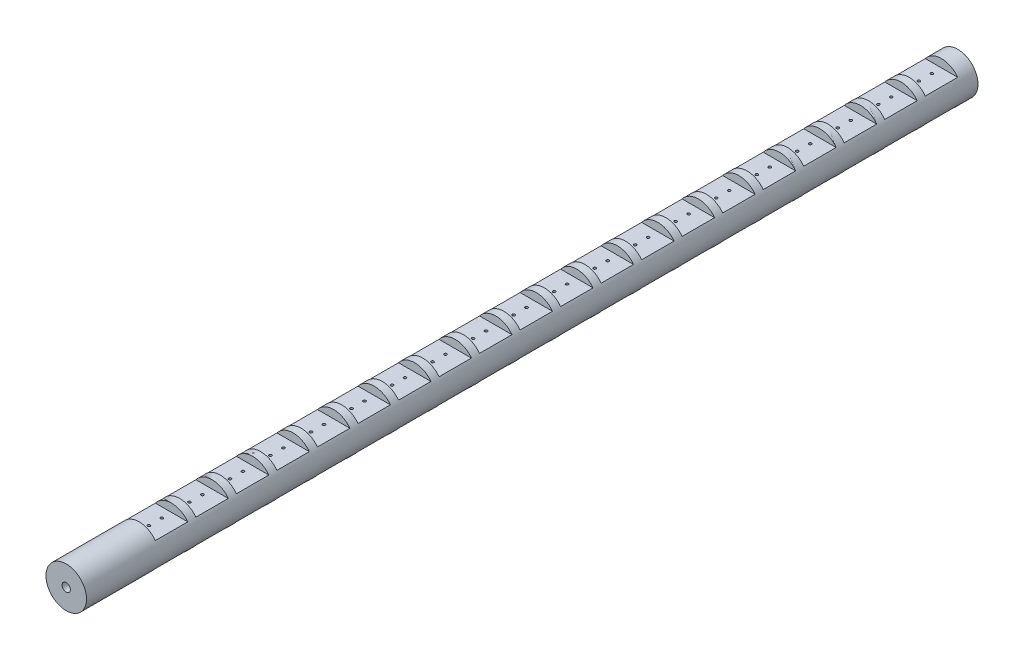
from build123d import *

# Parameters (mm, degrees)
SKETCH1_R                  = 25
BOSS_EXTRUDE1_DEPTH        = 1100
M12_TAPPED_HOLE1_D         = 10.2
M12_TAPPED_HOLE1_DEPTH     = 29.25
M12_TAPPED_HOLE1_TIP       = 3.064389157
SKETCH3_R                  = 10
CUT_EXTRUDE1_DEPTH         = 484
CUT_EXTRUDE2_START         = -15
SKETCH4_W                  = 50
SKETCH4_H                  = 40
CUT_EXTRUDE2_DEPTH         = 484
M4_TAPPED_HOLE1_AT_2_COUNT = 2
M4_TAPPED_HOLE1_AT_2_PITCH = 16
LPATTERN1_COUNT            = 20
LPATTERN1_PITCH            = 50
MIRROR1_START              = -15
MIRROR1_COPY_2_SKETCH_W    = 50
MIRROR1_COPY_2_SKETCH_H    = 40
MIRROR1_COPY_2_DEPTH       = 484
MIRROR1_COPY_3_SKETCH_W    = 50
MIRROR1_COPY_3_SKETCH_H    = 40
MIRROR1_COPY_3_DEPTH       = 484
MIRROR1_COPY_4_SKETCH_W    = 50
MIRROR1_COPY_4_SKETCH_H    = 40
MIRROR1_COPY_4_DEPTH       = 484
MIRROR1_COPY_5_SKETCH_W    = 50
MIRROR1_COPY_5_SKETCH_H    = 40
MIRROR1_COPY_5_DEPTH       = 484
MIRROR1_COPY_6_SKETCH_W    = 50
MIRROR1_COPY_6_SKETCH_H    = 40
MIRROR1_COPY_6_DEPTH       = 484
MIRROR1_COPY_7_SKETCH_W    = 50
MIRROR1_COPY_7_SKETCH_H    = 40
MIRROR1_COPY_7_DEPTH       = 484
MIRROR1_COPY_8_SKETCH_W    = 50
MIRROR1_COPY_8_SKETCH_H    = 40
MIRROR1_COPY_8_DEPTH       = 484
MIRROR1_COPY_9_SKETCH_W    = 50
MIRROR1_COPY_9_SKETCH_H    = 40
MIRROR1_COPY_9_DEPTH       = 484
MIRROR1_COPY_10_SKETCH_W   = 50
MIRROR1_COPY_10_SKETCH_H   = 40
MIRROR1_COPY_10_DEPTH      = 484
MIRROR1_COPY_11_SKETCH_W   = 50
MIRROR1_COPY_11_SKETCH_H   = 40
MIRROR1_COPY_11_DEPTH      = 484
MIRROR1_COPY_12_SKETCH_W   = 50
MIRROR1_COPY_12_SKETCH_H   = 40
MIRROR1_COPY_12_DEPTH      = 484
MIRROR1_COPY_13_SKETCH_W   = 50
MIRROR1_COPY_13_SKETCH_H   = 40
MIRROR1_COPY_13_DEPTH      = 484
MIRROR1_COPY_14_SKETCH_W   = 50
MIRROR1_COPY_14_SKETCH_H   = 40
MIRROR1_COPY_14_DEPTH      = 484
MIRROR1_COPY_15_SKETCH_W   = 50
MIRROR1_COPY_15_SKETCH_H   = 40
MIRROR1_COPY_15_DEPTH      = 484
MIRROR1_COPY_16_SKETCH_W   = 50
MIRROR1_COPY_16_SKETCH_H   = 40
MIRROR1_COPY_16_DEPTH      = 484
MIRROR1_COPY_17_SKETCH_W   = 50
MIRROR1_COPY_17_SKETCH_H   = 40
MIRROR1_COPY_17_DEPTH      = 484
MIRROR1_COPY_18_SKETCH_W   = 50
MIRROR1_COPY_18_SKETCH_H   = 40
MIRROR1_COPY_18_DEPTH      = 484
MIRROR1_COPY_19_SKETCH_W   = 50
MIRROR1_COPY_19_SKETCH_H   = 40
MIRROR1_COPY_19_DEPTH      = 484
MIRROR1_COPY_20_SKETCH_W   = 50
MIRROR1_COPY_20_SKETCH_H   = 40
MIRROR1_COPY_20_DEPTH      = 484
M4_TAPPED_HOLE2_D          = 3.3
M4_TAPPED_HOLE2_DEPTH      = 10.1
M4_TAPPED_HOLE2_TIP        = 0.991420021


with BuildPart() as part:
    # Sketch1 → Boss-Extrude1 (new body)
    with BuildSketch(Plane.XY):
        Circle(SKETCH1_R)
    extrude(amount=BOSS_EXTRUDE1_DEPTH)

    # M12 Tapped Hole1
    with Locations(Plane.XY.offset(1100)):
        with Locations((0, 0)):
            Hole(M12_TAPPED_HOLE1_D / 2, depth=M12_TAPPED_HOLE1_DEPTH)
            with Locations((0, 0, -(M12_TAPPED_HOLE1_DEPTH + M12_TAPPED_HOLE1_TIP / 2))):  # 118° drill point
                Cone(0, M12_TAPPED_HOLE1_D / 2, M12_TAPPED_HOLE1_TIP, mode=Mode.SUBTRACT)

    # Sketch3 → Cut-Extrude1 (cut)
    with BuildSketch(Plane(origin=(0, 0, 0), x_dir=(-1, 0, 0), z_dir=(0, 0, -1))):
        Circle(SKETCH3_R)
    extrude(amount=-CUT_EXTRUDE1_DEPTH, mode=Mode.SUBTRACT)

    # Sketch4 → Cut-Extrude2 (cut)
    with BuildSketch(Plane(origin=(0, 0, 0), x_dir=(1, 0, 0), z_dir=(0, 1, 0)).offset(CUT_EXTRUDE2_START)):
        with Locations((0, -40)):
            Rectangle(SKETCH4_W, SKETCH4_H)
    cut_extrude2 = extrude(amount=-CUT_EXTRUDE2_DEPTH, mode=Mode.SUBTRACT)

    # Sketch6 → M4 Tapped Hole1 (revolve, cut)
    with BuildSketch(Plane(origin=(0, -15, 48), x_dir=(0, 0, -1), z_dir=(1, 0, 0))):
        Polygon((0, 0), (0, 11.091420021), (1.65, 10.1), (1.65, 0), align=None)
    m4_tapped_hole1 = revolve(axis=Axis((0, -21.35, 48), (0, 1, 0)), mode=Mode.SUBTRACT)

    # M4 Tapped Hole1 at 2: M4 Tapped Hole1 ×2
    with Locations(*[(0, 0, -i * M4_TAPPED_HOLE1_AT_2_PITCH) for i in range(1, M4_TAPPED_HOLE1_AT_2_COUNT)]):
        add(m4_tapped_hole1, mode=Mode.SUBTRACT)

    # LPattern1: Cut-Extrude2, M4 Tapped Hole1 ×20
    with Locations(*[(0, 0, i * LPATTERN1_PITCH) for i in range(1, LPATTERN1_COUNT)]):
        add(cut_extrude2, mode=Mode.SUBTRACT)
        add(m4_tapped_hole1, mode=Mode.SUBTRACT)

    # LPattern1 copy 1 sketch → LPattern1 copy 1 (revolve, cut)
    with BuildSketch(Plane(origin=(0, -15, 82), x_dir=(0, 0, -1), z_dir=(1, 0, 0))):
        Polygon((0, 0), (0, 11.091420021), (1.65, 10.1), (1.65, 0), align=None)
    revolve(axis=Axis((0, -21.35, 82), (0, 1, 0)), mode=Mode.SUBTRACT)

    # LPattern1 copy 2 sketch → LPattern1 copy 2 (revolve, cut)
    with BuildSketch(Plane(origin=(0, -15, 132), x_dir=(0, 0, -1), z_dir=(1, 0, 0))):
        Polygon((0, 0), (0, 11.091420021), (1.65, 10.1), (1.65, 0), align=None)
    revolve(axis=Axis((0, -21.35, 132), (0, 1, 0)), mode=Mode.SUBTRACT)

    # LPattern1 copy 3 sketch → LPattern1 copy 3 (revolve, cut)
    with BuildSketch(Plane(origin=(0, -15, 182), x_dir=(0, 0, -1), z_dir=(1, 0, 0))):
        Polygon((0, 0), (0, 11.091420021), (1.65, 10.1), (1.65, 0), align=None)
    revolve(axis=Axis((0, -21.35, 182), (0, 1, 0)), mode=Mode.SUBTRACT)

    # LPattern1 copy 4 sketch → LPattern1 copy 4 (revolve, cut)
    with BuildSketch(Plane(origin=(0, -15, 232), x_dir=(0, 0, -1), z_dir=(1, 0, 0))):
        Polygon((0, 0), (0, 11.091420021), (1.65, 10.1), (1.65, 0), align=None)
    revolve(axis=Axis((0, -21.35, 232), (0, 1, 0)), mode=Mode.SUBTRACT)

    # LPattern1 copy 5 sketch → LPattern1 copy 5 (revolve, cut)
    with BuildSketch(Plane(origin=(0, -15, 282), x_dir=(0, 0, -1), z_dir=(1, 0, 0))):
        Polygon((0, 0), (0, 11.091420021), (1.65, 10.1), (1.65, 0), align=None)
    revolve(axis=Axis((0, -21.35, 282), (0, 1, 0)), mode=Mode.SUBTRACT)

    # LPattern1 copy 6 sketch → LPattern1 copy 6 (revolve, cut)
    with BuildSketch(Plane(origin=(0, -15, 332), x_dir=(0, 0, -1), z_dir=(1, 0, 0))):
        Polygon((0, 0), (0, 11.091420021), (1.65, 10.1), (1.65, 0), align=None)
    revolve(axis=Axis((0, -21.35, 332), (0, 1, 0)), mode=Mode.SUBTRACT)

    # LPattern1 copy 7 sketch → LPattern1 copy 7 (revolve, cut)
    with BuildSketch(Plane(origin=(0, -15, 382), x_dir=(0, 0, -1), z_dir=(1, 0, 0))):
        Polygon((0, 0), (0, 11.091420021), (1.65, 10.1), (1.65, 0), align=None)
    revolve(axis=Axis((0, -21.35, 382), (0, 1, 0)), mode=Mode.SUBTRACT)

    # LPattern1 copy 8 sketch → LPattern1 copy 8 (revolve, cut)
    with BuildSketch(Plane(origin=(0, -15, 432), x_dir=(0, 0, -1), z_dir=(1, 0, 0))):
        Polygon((0, 0), (0, 11.091420021), (1.65, 10.1), (1.65, 0), align=None)
    revolve(axis=Axis((0, -21.35, 432), (0, 1, 0)), mode=Mode.SUBTRACT)

    # LPattern1 copy 9 sketch → LPattern1 copy 9 (revolve, cut)
    with BuildSketch(Plane(origin=(0, -15, 482), x_dir=(0, 0, -1), z_dir=(1, 0, 0))):
        Polygon((0, 0), (0, 11.091420021), (1.65, 10.1), (1.65, 0), align=None)
    revolve(axis=Axis((0, -21.35, 482), (0, 1, 0)), mode=Mode.SUBTRACT)

    # LPattern1 copy 10 sketch → LPattern1 copy 10 (revolve, cut)
    with BuildSketch(Plane(origin=(0, -15, 532), x_dir=(0, 0, -1), z_dir=(1, 0, 0))):
        Polygon((0, 0), (0, 11.091420021), (1.65, 10.1), (1.65, 0), align=None)
    revolve(axis=Axis((0, -21.35, 532), (0, 1, 0)), mode=Mode.SUBTRACT)

    # LPattern1 copy 11 sketch → LPattern1 copy 11 (revolve, cut)
    with BuildSketch(Plane(origin=(0, -15, 582), x_dir=(0, 0, -1), z_dir=(1, 0, 0))):
        Polygon((0, 0), (0, 11.091420021), (1.65, 10.1), (1.65, 0), align=None)
    revolve(axis=Axis((0, -21.35, 582), (0, 1, 0)), mode=Mode.SUBTRACT)

    # LPattern1 copy 12 sketch → LPattern1 copy 12 (revolve, cut)
    with BuildSketch(Plane(origin=(0, -15, 632), x_dir=(0, 0, -1), z_dir=(1, 0, 0))):
        Polygon((0, 0), (0, 11.091420021), (1.65, 10.1), (1.65, 0), align=None)
    revolve(axis=Axis((0, -21.35, 632), (0, 1, 0)), mode=Mode.SUBTRACT)

    # LPattern1 copy 13 sketch → LPattern1 copy 13 (revolve, cut)
    with BuildSketch(Plane(origin=(0, -15, 682), x_dir=(0, 0, -1), z_dir=(1, 0, 0))):
        Polygon((0, 0), (0, 11.091420021), (1.65, 10.1), (1.65, 0), align=None)
    revolve(axis=Axis((0, -21.35, 682), (0, 1, 0)), mode=Mode.SUBTRACT)

    # LPattern1 copy 14 sketch → LPattern1 copy 14 (revolve, cut)
    with BuildSketch(Plane(origin=(0, -15, 732), x_dir=(0, 0, -1), z_dir=(1, 0, 0))):
        Polygon((0, 0), (0, 11.091420021), (1.65, 10.1), (1.65, 0), align=None)
    revolve(axis=Axis((0, -21.35, 732), (0, 1, 0)), mode=Mode.SUBTRACT)

    # LPattern1 copy 15 sketch → LPattern1 copy 15 (revolve, cut)
    with BuildSketch(Plane(origin=(0, -15, 782), x_dir=(0, 0, -1), z_dir=(1, 0, 0))):
        Polygon((0, 0), (0, 11.091420021), (1.65, 10.1), (1.65, 0), align=None)
    revolve(axis=Axis((0, -21.35, 782), (0, 1, 0)), mode=Mode.SUBTRACT)

    # LPattern1 copy 16 sketch → LPattern1 copy 16 (revolve, cut)
    with BuildSketch(Plane(origin=(0, -15, 832), x_dir=(0, 0, -1), z_dir=(1, 0, 0))):
        Polygon((0, 0), (0, 11.091420021), (1.65, 10.1), (1.65, 0), align=None)
    revolve(axis=Axis((0, -21.35, 832), (0, 1, 0)), mode=Mode.SUBTRACT)

    # LPattern1 copy 17 sketch → LPattern1 copy 17 (revolve, cut)
    with BuildSketch(Plane(origin=(0, -15, 882), x_dir=(0, 0, -1), z_dir=(1, 0, 0))):
        Polygon((0, 0), (0, 11.091420021), (1.65, 10.1), (1.65, 0), align=None)
    revolve(axis=Axis((0, -21.35, 882), (0, 1, 0)), mode=Mode.SUBTRACT)

    # LPattern1 copy 18 sketch → LPattern1 copy 18 (revolve, cut)
    with BuildSketch(Plane(origin=(0, -15, 932), x_dir=(0, 0, -1), z_dir=(1, 0, 0))):
        Polygon((0, 0), (0, 11.091420021), (1.65, 10.1), (1.65, 0), align=None)
    revolve(axis=Axis((0, -21.35, 932), (0, 1, 0)), mode=Mode.SUBTRACT)

    # LPattern1 copy 19 sketch → LPattern1 copy 19 (revolve, cut)
    with BuildSketch(Plane(origin=(0, -15, 982), x_dir=(0, 0, -1), z_dir=(1, 0, 0))):
        Polygon((0, 0), (0, 11.091420021), (1.65, 10.1), (1.65, 0), align=None)
    revolve(axis=Axis((0, -21.35, 982), (0, 1, 0)), mode=Mode.SUBTRACT)

    # Mirror1: Cut-Extrude2, M4 Tapped Hole1 across plane
    add(cut_extrude2.mirror(Plane.ZX), mode=Mode.SUBTRACT)
    add(m4_tapped_hole1.mirror(Plane.ZX), mode=Mode.SUBTRACT)

    # Mirror1 copy 1 sketch → Mirror1 copy 1 (revolve, cut)
    with BuildSketch(Plane(origin=(0, 15, 32), x_dir=(0, 0, -1), z_dir=(1, 0, 0))):
        Polygon((0, 0), (0, -11.091420021), (1.65, -10.1), (1.65, 0), align=None)
    revolve(axis=Axis((0, 21.35, 32), (0, 1, 0)), mode=Mode.SUBTRACT)

    # Mirror1 copy 2 sketch → Mirror1 copy 2 (cut)
    with BuildSketch(Plane(origin=(0, 0, 50), x_dir=(1, 0, 0), z_dir=(0, -1, 0)).offset(MIRROR1_START)):
        with Locations((0, 40)):
            Rectangle(MIRROR1_COPY_2_SKETCH_W, MIRROR1_COPY_2_SKETCH_H)
    extrude(amount=-MIRROR1_COPY_2_DEPTH, mode=Mode.SUBTRACT)

    # Mirror1 copy 3 sketch → Mirror1 copy 3 (cut)
    with BuildSketch(Plane(origin=(0, 0, 100), x_dir=(1, 0, 0), z_dir=(0, -1, 0)).offset(MIRROR1_START)):
        with Locations((0, 40)):
            Rectangle(MIRROR1_COPY_3_SKETCH_W, MIRROR1_COPY_3_SKETCH_H)
    extrude(amount=-MIRROR1_COPY_3_DEPTH, mode=Mode.SUBTRACT)

    # Mirror1 copy 4 sketch → Mirror1 copy 4 (cut)
    with BuildSketch(Plane(origin=(0, 0, 150), x_dir=(1, 0, 0), z_dir=(0, -1, 0)).offset(MIRROR1_START)):
        with Locations((0, 40)):
            Rectangle(MIRROR1_COPY_4_SKETCH_W, MIRROR1_COPY_4_SKETCH_H)
    extrude(amount=-MIRROR1_COPY_4_DEPTH, mode=Mode.SUBTRACT)

    # Mirror1 copy 5 sketch → Mirror1 copy 5 (cut)
    with BuildSketch(Plane(origin=(0, 0, 200), x_dir=(1, 0, 0), z_dir=(0, -1, 0)).offset(MIRROR1_START)):
        with Locations((0, 40)):
            Rectangle(MIRROR1_COPY_5_SKETCH_W, MIRROR1_COPY_5_SKETCH_H)
    extrude(amount=-MIRROR1_COPY_5_DEPTH, mode=Mode.SUBTRACT)

    # Mirror1 copy 6 sketch → Mirror1 copy 6 (cut)
    with BuildSketch(Plane(origin=(0, 0, 250), x_dir=(1, 0, 0), z_dir=(0, -1, 0)).offset(MIRROR1_START)):
        with Locations((0, 40)):
            Rectangle(MIRROR1_COPY_6_SKETCH_W, MIRROR1_COPY_6_SKETCH_H)
    extrude(amount=-MIRROR1_COPY_6_DEPTH, mode=Mode.SUBTRACT)

    # Mirror1 copy 7 sketch → Mirror1 copy 7 (cut)
    with BuildSketch(Plane(origin=(0, 0, 300), x_dir=(1, 0, 0), z_dir=(0, -1, 0)).offset(MIRROR1_START)):
        with Locations((0, 40)):
            Rectangle(MIRROR1_COPY_7_SKETCH_W, MIRROR1_COPY_7_SKETCH_H)
    extrude(amount=-MIRROR1_COPY_7_DEPTH, mode=Mode.SUBTRACT)

    # Mirror1 copy 8 sketch → Mirror1 copy 8 (cut)
    with BuildSketch(Plane(origin=(0, 0, 350), x_dir=(1, 0, 0), z_dir=(0, -1, 0)).offset(MIRROR1_START)):
        with Locations((0, 40)):
            Rectangle(MIRROR1_COPY_8_SKETCH_W, MIRROR1_COPY_8_SKETCH_H)
    extrude(amount=-MIRROR1_COPY_8_DEPTH, mode=Mode.SUBTRACT)

    # Mirror1 copy 9 sketch → Mirror1 copy 9 (cut)
    with BuildSketch(Plane(origin=(0, 0, 400), x_dir=(1, 0, 0), z_dir=(0, -1, 0)).offset(MIRROR1_START)):
        with Locations((0, 40)):
            Rectangle(MIRROR1_COPY_9_SKETCH_W, MIRROR1_COPY_9_SKETCH_H)
    extrude(amount=-MIRROR1_COPY_9_DEPTH, mode=Mode.SUBTRACT)

    # Mirror1 copy 10 sketch → Mirror1 copy 10 (cut)
    with BuildSketch(Plane(origin=(0, 0, 450), x_dir=(1, 0, 0), z_dir=(0, -1, 0)).offset(MIRROR1_START)):
        with Locations((0, 40)):
            Rectangle(MIRROR1_COPY_10_SKETCH_W, MIRROR1_COPY_10_SKETCH_H)
    extrude(amount=-MIRROR1_COPY_10_DEPTH, mode=Mode.SUBTRACT)

    # Mirror1 copy 11 sketch → Mirror1 copy 11 (cut)
    with BuildSketch(Plane(origin=(0, 0, 500), x_dir=(1, 0, 0), z_dir=(0, -1, 0)).offset(MIRROR1_START)):
        with Locations((0, 40)):
            Rectangle(MIRROR1_COPY_11_SKETCH_W, MIRROR1_COPY_11_SKETCH_H)
    extrude(amount=-MIRROR1_COPY_11_DEPTH, mode=Mode.SUBTRACT)

    # Mirror1 copy 12 sketch → Mirror1 copy 12 (cut)
    with BuildSketch(Plane(origin=(0, 0, 550), x_dir=(1, 0, 0), z_dir=(0, -1, 0)).offset(MIRROR1_START)):
        with Locations((0, 40)):
            Rectangle(MIRROR1_COPY_12_SKETCH_W, MIRROR1_COPY_12_SKETCH_H)
    extrude(amount=-MIRROR1_COPY_12_DEPTH, mode=Mode.SUBTRACT)

    # Mirror1 copy 13 sketch → Mirror1 copy 13 (cut)
    with BuildSketch(Plane(origin=(0, 0, 600), x_dir=(1, 0, 0), z_dir=(0, -1, 0)).offset(MIRROR1_START)):
        with Locations((0, 40)):
            Rectangle(MIRROR1_COPY_13_SKETCH_W, MIRROR1_COPY_13_SKETCH_H)
    extrude(amount=-MIRROR1_COPY_13_DEPTH, mode=Mode.SUBTRACT)

    # Mirror1 copy 14 sketch → Mirror1 copy 14 (cut)
    with BuildSketch(Plane(origin=(0, 0, 650), x_dir=(1, 0, 0), z_dir=(0, -1, 0)).offset(MIRROR1_START)):
        with Locations((0, 40)):
            Rectangle(MIRROR1_COPY_14_SKETCH_W, MIRROR1_COPY_14_SKETCH_H)
    extrude(amount=-MIRROR1_COPY_14_DEPTH, mode=Mode.SUBTRACT)

    # Mirror1 copy 15 sketch → Mirror1 copy 15 (cut)
    with BuildSketch(Plane(origin=(0, 0, 700), x_dir=(1, 0, 0), z_dir=(0, -1, 0)).offset(MIRROR1_START)):
        with Locations((0, 40)):
            Rectangle(MIRROR1_COPY_15_SKETCH_W, MIRROR1_COPY_15_SKETCH_H)
    extrude(amount=-MIRROR1_COPY_15_DEPTH, mode=Mode.SUBTRACT)

    # Mirror1 copy 16 sketch → Mirror1 copy 16 (cut)
    with BuildSketch(Plane(origin=(0, 0, 750), x_dir=(1, 0, 0), z_dir=(0, -1, 0)).offset(MIRROR1_START)):
        with Locations((0, 40)):
            Rectangle(MIRROR1_COPY_16_SKETCH_W, MIRROR1_COPY_16_SKETCH_H)
    extrude(amount=-MIRROR1_COPY_16_DEPTH, mode=Mode.SUBTRACT)

    # Mirror1 copy 17 sketch → Mirror1 copy 17 (cut)
    with BuildSketch(Plane(origin=(0, 0, 800), x_dir=(1, 0, 0), z_dir=(0, -1, 0)).offset(MIRROR1_START)):
        with Locations((0, 40)):
            Rectangle(MIRROR1_COPY_17_SKETCH_W, MIRROR1_COPY_17_SKETCH_H)
    extrude(amount=-MIRROR1_COPY_17_DEPTH, mode=Mode.SUBTRACT)

    # Mirror1 copy 18 sketch → Mirror1 copy 18 (cut)
    with BuildSketch(Plane(origin=(0, 0, 850), x_dir=(1, 0, 0), z_dir=(0, -1, 0)).offset(MIRROR1_START)):
        with Locations((0, 40)):
            Rectangle(MIRROR1_COPY_18_SKETCH_W, MIRROR1_COPY_18_SKETCH_H)
    extrude(amount=-MIRROR1_COPY_18_DEPTH, mode=Mode.SUBTRACT)

    # Mirror1 copy 19 sketch → Mirror1 copy 19 (cut)
    with BuildSketch(Plane(origin=(0, 0, 900), x_dir=(1, 0, 0), z_dir=(0, -1, 0)).offset(MIRROR1_START)):
        with Locations((0, 40)):
            Rectangle(MIRROR1_COPY_19_SKETCH_W, MIRROR1_COPY_19_SKETCH_H)
    extrude(amount=-MIRROR1_COPY_19_DEPTH, mode=Mode.SUBTRACT)

    # Mirror1 copy 20 sketch → Mirror1 copy 20 (cut)
    with BuildSketch(Plane(origin=(0, 0, 950), x_dir=(1, 0, 0), z_dir=(0, -1, 0)).offset(MIRROR1_START)):
        with Locations((0, 40)):
            Rectangle(MIRROR1_COPY_20_SKETCH_W, MIRROR1_COPY_20_SKETCH_H)
    extrude(amount=-MIRROR1_COPY_20_DEPTH, mode=Mode.SUBTRACT)

    # Mirror1 copy 21 sketch → Mirror1 copy 21 (revolve, cut)
    with BuildSketch(Plane(origin=(0, 15, 98), x_dir=(0, 0, -1), z_dir=(1, 0, 0))):
        Polygon((0, 0), (0, -11.091420021), (1.65, -10.1), (1.65, 0), align=None)
    revolve(axis=Axis((0, 21.35, 98), (0, 1, 0)), mode=Mode.SUBTRACT)

    # Mirror1 copy 22 sketch → Mirror1 copy 22 (revolve, cut)
    with BuildSketch(Plane(origin=(0, 15, 148), x_dir=(0, 0, -1), z_dir=(1, 0, 0))):
        Polygon((0, 0), (0, -11.091420021), (1.65, -10.1), (1.65, 0), align=None)
    revolve(axis=Axis((0, 21.35, 148), (0, 1, 0)), mode=Mode.SUBTRACT)

    # Mirror1 copy 23 sketch → Mirror1 copy 23 (revolve, cut)
    with BuildSketch(Plane(origin=(0, 15, 198), x_dir=(0, 0, -1), z_dir=(1, 0, 0))):
        Polygon((0, 0), (0, -11.091420021), (1.65, -10.1), (1.65, 0), align=None)
    revolve(axis=Axis((0, 21.35, 198), (0, 1, 0)), mode=Mode.SUBTRACT)

    # Mirror1 copy 24 sketch → Mirror1 copy 24 (revolve, cut)
    with BuildSketch(Plane(origin=(0, 15, 248), x_dir=(0, 0, -1), z_dir=(1, 0, 0))):
        Polygon((0, 0), (0, -11.091420021), (1.65, -10.1), (1.65, 0), align=None)
    revolve(axis=Axis((0, 21.35, 248), (0, 1, 0)), mode=Mode.SUBTRACT)

    # Mirror1 copy 25 sketch → Mirror1 copy 25 (revolve, cut)
    with BuildSketch(Plane(origin=(0, 15, 298), x_dir=(0, 0, -1), z_dir=(1, 0, 0))):
        Polygon((0, 0), (0, -11.091420021), (1.65, -10.1), (1.65, 0), align=None)
    revolve(axis=Axis((0, 21.35, 298), (0, 1, 0)), mode=Mode.SUBTRACT)

    # Mirror1 copy 26 sketch → Mirror1 copy 26 (revolve, cut)
    with BuildSketch(Plane(origin=(0, 15, 348), x_dir=(0, 0, -1), z_dir=(1, 0, 0))):
        Polygon((0, 0), (0, -11.091420021), (1.65, -10.1), (1.65, 0), align=None)
    revolve(axis=Axis((0, 21.35, 348), (0, 1, 0)), mode=Mode.SUBTRACT)

    # Mirror1 copy 27 sketch → Mirror1 copy 27 (revolve, cut)
    with BuildSketch(Plane(origin=(0, 15, 398), x_dir=(0, 0, -1), z_dir=(1, 0, 0))):
        Polygon((0, 0), (0, -11.091420021), (1.65, -10.1), (1.65, 0), align=None)
    revolve(axis=Axis((0, 21.35, 398), (0, 1, 0)), mode=Mode.SUBTRACT)

    # Mirror1 copy 28 sketch → Mirror1 copy 28 (revolve, cut)
    with BuildSketch(Plane(origin=(0, 15, 448), x_dir=(0, 0, -1), z_dir=(1, 0, 0))):
        Polygon((0, 0), (0, -11.091420021), (1.65, -10.1), (1.65, 0), align=None)
    revolve(axis=Axis((0, 21.35, 448), (0, 1, 0)), mode=Mode.SUBTRACT)

    # Mirror1 copy 29 sketch → Mirror1 copy 29 (revolve, cut)
    with BuildSketch(Plane(origin=(0, 15, 498), x_dir=(0, 0, -1), z_dir=(1, 0, 0))):
        Polygon((0, 0), (0, -11.091420021), (1.65, -10.1), (1.65, 0), align=None)
    revolve(axis=Axis((0, 21.35, 498), (0, 1, 0)), mode=Mode.SUBTRACT)

    # Mirror1 copy 30 sketch → Mirror1 copy 30 (revolve, cut)
    with BuildSketch(Plane(origin=(0, 15, 548), x_dir=(0, 0, -1), z_dir=(1, 0, 0))):
        Polygon((0, 0), (0, -11.091420021), (1.65, -10.1), (1.65, 0), align=None)
    revolve(axis=Axis((0, 21.35, 548), (0, 1, 0)), mode=Mode.SUBTRACT)

    # Mirror1 copy 31 sketch → Mirror1 copy 31 (revolve, cut)
    with BuildSketch(Plane(origin=(0, 15, 598), x_dir=(0, 0, -1), z_dir=(1, 0, 0))):
        Polygon((0, 0), (0, -11.091420021), (1.65, -10.1), (1.65, 0), align=None)
    revolve(axis=Axis((0, 21.35, 598), (0, 1, 0)), mode=Mode.SUBTRACT)

    # Mirror1 copy 32 sketch → Mirror1 copy 32 (revolve, cut)
    with BuildSketch(Plane(origin=(0, 15, 648), x_dir=(0, 0, -1), z_dir=(1, 0, 0))):
        Polygon((0, 0), (0, -11.091420021), (1.65, -10.1), (1.65, 0), align=None)
    revolve(axis=Axis((0, 21.35, 648), (0, 1, 0)), mode=Mode.SUBTRACT)

    # Mirror1 copy 33 sketch → Mirror1 copy 33 (revolve, cut)
    with BuildSketch(Plane(origin=(0, 15, 698), x_dir=(0, 0, -1), z_dir=(1, 0, 0))):
        Polygon((0, 0), (0, -11.091420021), (1.65, -10.1), (1.65, 0), align=None)
    revolve(axis=Axis((0, 21.35, 698), (0, 1, 0)), mode=Mode.SUBTRACT)

    # Mirror1 copy 34 sketch → Mirror1 copy 34 (revolve, cut)
    with BuildSketch(Plane(origin=(0, 15, 748), x_dir=(0, 0, -1), z_dir=(1, 0, 0))):
        Polygon((0, 0), (0, -11.091420021), (1.65, -10.1), (1.65, 0), align=None)
    revolve(axis=Axis((0, 21.35, 748), (0, 1, 0)), mode=Mode.SUBTRACT)

    # Mirror1 copy 35 sketch → Mirror1 copy 35 (revolve, cut)
    with BuildSketch(Plane(origin=(0, 15, 798), x_dir=(0, 0, -1), z_dir=(1, 0, 0))):
        Polygon((0, 0), (0, -11.091420021), (1.65, -10.1), (1.65, 0), align=None)
    revolve(axis=Axis((0, 21.35, 798), (0, 1, 0)), mode=Mode.SUBTRACT)

    # Mirror1 copy 36 sketch → Mirror1 copy 36 (revolve, cut)
    with BuildSketch(Plane(origin=(0, 15, 848), x_dir=(0, 0, -1), z_dir=(1, 0, 0))):
        Polygon((0, 0), (0, -11.091420021), (1.65, -10.1), (1.65, 0), align=None)
    revolve(axis=Axis((0, 21.35, 848), (0, 1, 0)), mode=Mode.SUBTRACT)

    # Mirror1 copy 37 sketch → Mirror1 copy 37 (revolve, cut)
    with BuildSketch(Plane(origin=(0, 15, 898), x_dir=(0, 0, -1), z_dir=(1, 0, 0))):
        Polygon((0, 0), (0, -11.091420021), (1.65, -10.1), (1.65, 0), align=None)
    revolve(axis=Axis((0, 21.35, 898), (0, 1, 0)), mode=Mode.SUBTRACT)

    # Mirror1 copy 38 sketch → Mirror1 copy 38 (revolve, cut)
    with BuildSketch(Plane(origin=(0, 15, 948), x_dir=(0, 0, -1), z_dir=(1, 0, 0))):
        Polygon((0, 0), (0, -11.091420021), (1.65, -10.1), (1.65, 0), align=None)
    revolve(axis=Axis((0, 21.35, 948), (0, 1, 0)), mode=Mode.SUBTRACT)

    # Mirror1 copy 39 sketch → Mirror1 copy 39 (revolve, cut)
    with BuildSketch(Plane(origin=(0, 15, 998), x_dir=(0, 0, -1), z_dir=(1, 0, 0))):
        Polygon((0, 0), (0, -11.091420021), (1.65, -10.1), (1.65, 0), align=None)
    revolve(axis=Axis((0, 21.35, 998), (0, 1, 0)), mode=Mode.SUBTRACT)

    # Mirror1 copy 40 sketch → Mirror1 copy 40 (revolve, cut)
    with BuildSketch(Plane(origin=(0, 15, 82), x_dir=(0, 0, -1), z_dir=(1, 0, 0))):
        Polygon((0, 0), (0, -11.091420021), (1.65, -10.1), (1.65, 0), align=None)
    revolve(axis=Axis((0, 21.35, 82), (0, 1, 0)), mode=Mode.SUBTRACT)

    # Mirror1 copy 41 sketch → Mirror1 copy 41 (revolve, cut)
    with BuildSketch(Plane(origin=(0, 15, 132), x_dir=(0, 0, -1), z_dir=(1, 0, 0))):
        Polygon((0, 0), (0, -11.091420021), (1.65, -10.1), (1.65, 0), align=None)
    revolve(axis=Axis((0, 21.35, 132), (0, 1, 0)), mode=Mode.SUBTRACT)

    # Mirror1 copy 42 sketch → Mirror1 copy 42 (revolve, cut)
    with BuildSketch(Plane(origin=(0, 15, 182), x_dir=(0, 0, -1), z_dir=(1, 0, 0))):
        Polygon((0, 0), (0, -11.091420021), (1.65, -10.1), (1.65, 0), align=None)
    revolve(axis=Axis((0, 21.35, 182), (0, 1, 0)), mode=Mode.SUBTRACT)

    # Mirror1 copy 43 sketch → Mirror1 copy 43 (revolve, cut)
    with BuildSketch(Plane(origin=(0, 15, 232), x_dir=(0, 0, -1), z_dir=(1, 0, 0))):
        Polygon((0, 0), (0, -11.091420021), (1.65, -10.1), (1.65, 0), align=None)
    revolve(axis=Axis((0, 21.35, 232), (0, 1, 0)), mode=Mode.SUBTRACT)

    # Mirror1 copy 44 sketch → Mirror1 copy 44 (revolve, cut)
    with BuildSketch(Plane(origin=(0, 15, 282), x_dir=(0, 0, -1), z_dir=(1, 0, 0))):
        Polygon((0, 0), (0, -11.091420021), (1.65, -10.1), (1.65, 0), align=None)
    revolve(axis=Axis((0, 21.35, 282), (0, 1, 0)), mode=Mode.SUBTRACT)

    # Mirror1 copy 45 sketch → Mirror1 copy 45 (revolve, cut)
    with BuildSketch(Plane(origin=(0, 15, 332), x_dir=(0, 0, -1), z_dir=(1, 0, 0))):
        Polygon((0, 0), (0, -11.091420021), (1.65, -10.1), (1.65, 0), align=None)
    revolve(axis=Axis((0, 21.35, 332), (0, 1, 0)), mode=Mode.SUBTRACT)

    # Mirror1 copy 46 sketch → Mirror1 copy 46 (revolve, cut)
    with BuildSketch(Plane(origin=(0, 15, 382), x_dir=(0, 0, -1), z_dir=(1, 0, 0))):
        Polygon((0, 0), (0, -11.091420021), (1.65, -10.1), (1.65, 0), align=None)
    revolve(axis=Axis((0, 21.35, 382), (0, 1, 0)), mode=Mode.SUBTRACT)

    # Mirror1 copy 47 sketch → Mirror1 copy 47 (revolve, cut)
    with BuildSketch(Plane(origin=(0, 15, 432), x_dir=(0, 0, -1), z_dir=(1, 0, 0))):
        Polygon((0, 0), (0, -11.091420021), (1.65, -10.1), (1.65, 0), align=None)
    revolve(axis=Axis((0, 21.35, 432), (0, 1, 0)), mode=Mode.SUBTRACT)

    # Mirror1 copy 48 sketch → Mirror1 copy 48 (revolve, cut)
    with BuildSketch(Plane(origin=(0, 15, 482), x_dir=(0, 0, -1), z_dir=(1, 0, 0))):
        Polygon((0, 0), (0, -11.091420021), (1.65, -10.1), (1.65, 0), align=None)
    revolve(axis=Axis((0, 21.35, 482), (0, 1, 0)), mode=Mode.SUBTRACT)

    # Mirror1 copy 49 sketch → Mirror1 copy 49 (revolve, cut)
    with BuildSketch(Plane(origin=(0, 15, 532), x_dir=(0, 0, -1), z_dir=(1, 0, 0))):
        Polygon((0, 0), (0, -11.091420021), (1.65, -10.1), (1.65, 0), align=None)
    revolve(axis=Axis((0, 21.35, 532), (0, 1, 0)), mode=Mode.SUBTRACT)

    # Mirror1 copy 50 sketch → Mirror1 copy 50 (revolve, cut)
    with BuildSketch(Plane(origin=(0, 15, 582), x_dir=(0, 0, -1), z_dir=(1, 0, 0))):
        Polygon((0, 0), (0, -11.091420021), (1.65, -10.1), (1.65, 0), align=None)
    revolve(axis=Axis((0, 21.35, 582), (0, 1, 0)), mode=Mode.SUBTRACT)

    # Mirror1 copy 51 sketch → Mirror1 copy 51 (revolve, cut)
    with BuildSketch(Plane(origin=(0, 15, 632), x_dir=(0, 0, -1), z_dir=(1, 0, 0))):
        Polygon((0, 0), (0, -11.091420021), (1.65, -10.1), (1.65, 0), align=None)
    revolve(axis=Axis((0, 21.35, 632), (0, 1, 0)), mode=Mode.SUBTRACT)

    # Mirror1 copy 52 sketch → Mirror1 copy 52 (revolve, cut)
    with BuildSketch(Plane(origin=(0, 15, 682), x_dir=(0, 0, -1), z_dir=(1, 0, 0))):
        Polygon((0, 0), (0, -11.091420021), (1.65, -10.1), (1.65, 0), align=None)
    revolve(axis=Axis((0, 21.35, 682), (0, 1, 0)), mode=Mode.SUBTRACT)

    # Mirror1 copy 53 sketch → Mirror1 copy 53 (revolve, cut)
    with BuildSketch(Plane(origin=(0, 15, 732), x_dir=(0, 0, -1), z_dir=(1, 0, 0))):
        Polygon((0, 0), (0, -11.091420021), (1.65, -10.1), (1.65, 0), align=None)
    revolve(axis=Axis((0, 21.35, 732), (0, 1, 0)), mode=Mode.SUBTRACT)

    # Mirror1 copy 54 sketch → Mirror1 copy 54 (revolve, cut)
    with BuildSketch(Plane(origin=(0, 15, 782), x_dir=(0, 0, -1), z_dir=(1, 0, 0))):
        Polygon((0, 0), (0, -11.091420021), (1.65, -10.1), (1.65, 0), align=None)
    revolve(axis=Axis((0, 21.35, 782), (0, 1, 0)), mode=Mode.SUBTRACT)

    # Mirror1 copy 55 sketch → Mirror1 copy 55 (revolve, cut)
    with BuildSketch(Plane(origin=(0, 15, 832), x_dir=(0, 0, -1), z_dir=(1, 0, 0))):
        Polygon((0, 0), (0, -11.091420021), (1.65, -10.1), (1.65, 0), align=None)
    revolve(axis=Axis((0, 21.35, 832), (0, 1, 0)), mode=Mode.SUBTRACT)

    # Mirror1 copy 56 sketch → Mirror1 copy 56 (revolve, cut)
    with BuildSketch(Plane(origin=(0, 15, 882), x_dir=(0, 0, -1), z_dir=(1, 0, 0))):
        Polygon((0, 0), (0, -11.091420021), (1.65, -10.1), (1.65, 0), align=None)
    revolve(axis=Axis((0, 21.35, 882), (0, 1, 0)), mode=Mode.SUBTRACT)

    # Mirror1 copy 57 sketch → Mirror1 copy 57 (revolve, cut)
    with BuildSketch(Plane(origin=(0, 15, 932), x_dir=(0, 0, -1), z_dir=(1, 0, 0))):
        Polygon((0, 0), (0, -11.091420021), (1.65, -10.1), (1.65, 0), align=None)
    revolve(axis=Axis((0, 21.35, 932), (0, 1, 0)), mode=Mode.SUBTRACT)

    # Mirror1 copy 58 sketch → Mirror1 copy 58 (revolve, cut)
    with BuildSketch(Plane(origin=(0, 15, 982), x_dir=(0, 0, -1), z_dir=(1, 0, 0))):
        Polygon((0, 0), (0, -11.091420021), (1.65, -10.1), (1.65, 0), align=None)
    revolve(axis=Axis((0, 21.35, 982), (0, 1, 0)), mode=Mode.SUBTRACT)

    # M4 Tapped Hole2
    with Locations(Plane(origin=(16.85938972, 0.513483951, 0), x_dir=(-1, 0, 0), z_dir=(0, 0, -1))):
        with Locations((0, 0), (34.574586024, -0.684645268)):
            Hole(M4_TAPPED_HOLE2_D / 2, depth=M4_TAPPED_HOLE2_DEPTH)
            with Locations((0, 0, -(M4_TAPPED_HOLE2_DEPTH + M4_TAPPED_HOLE2_TIP / 2))):  # 118° drill point
                Cone(0, M4_TAPPED_HOLE2_D / 2, M4_TAPPED_HOLE2_TIP, mode=Mode.SUBTRACT)


solid = part.part
